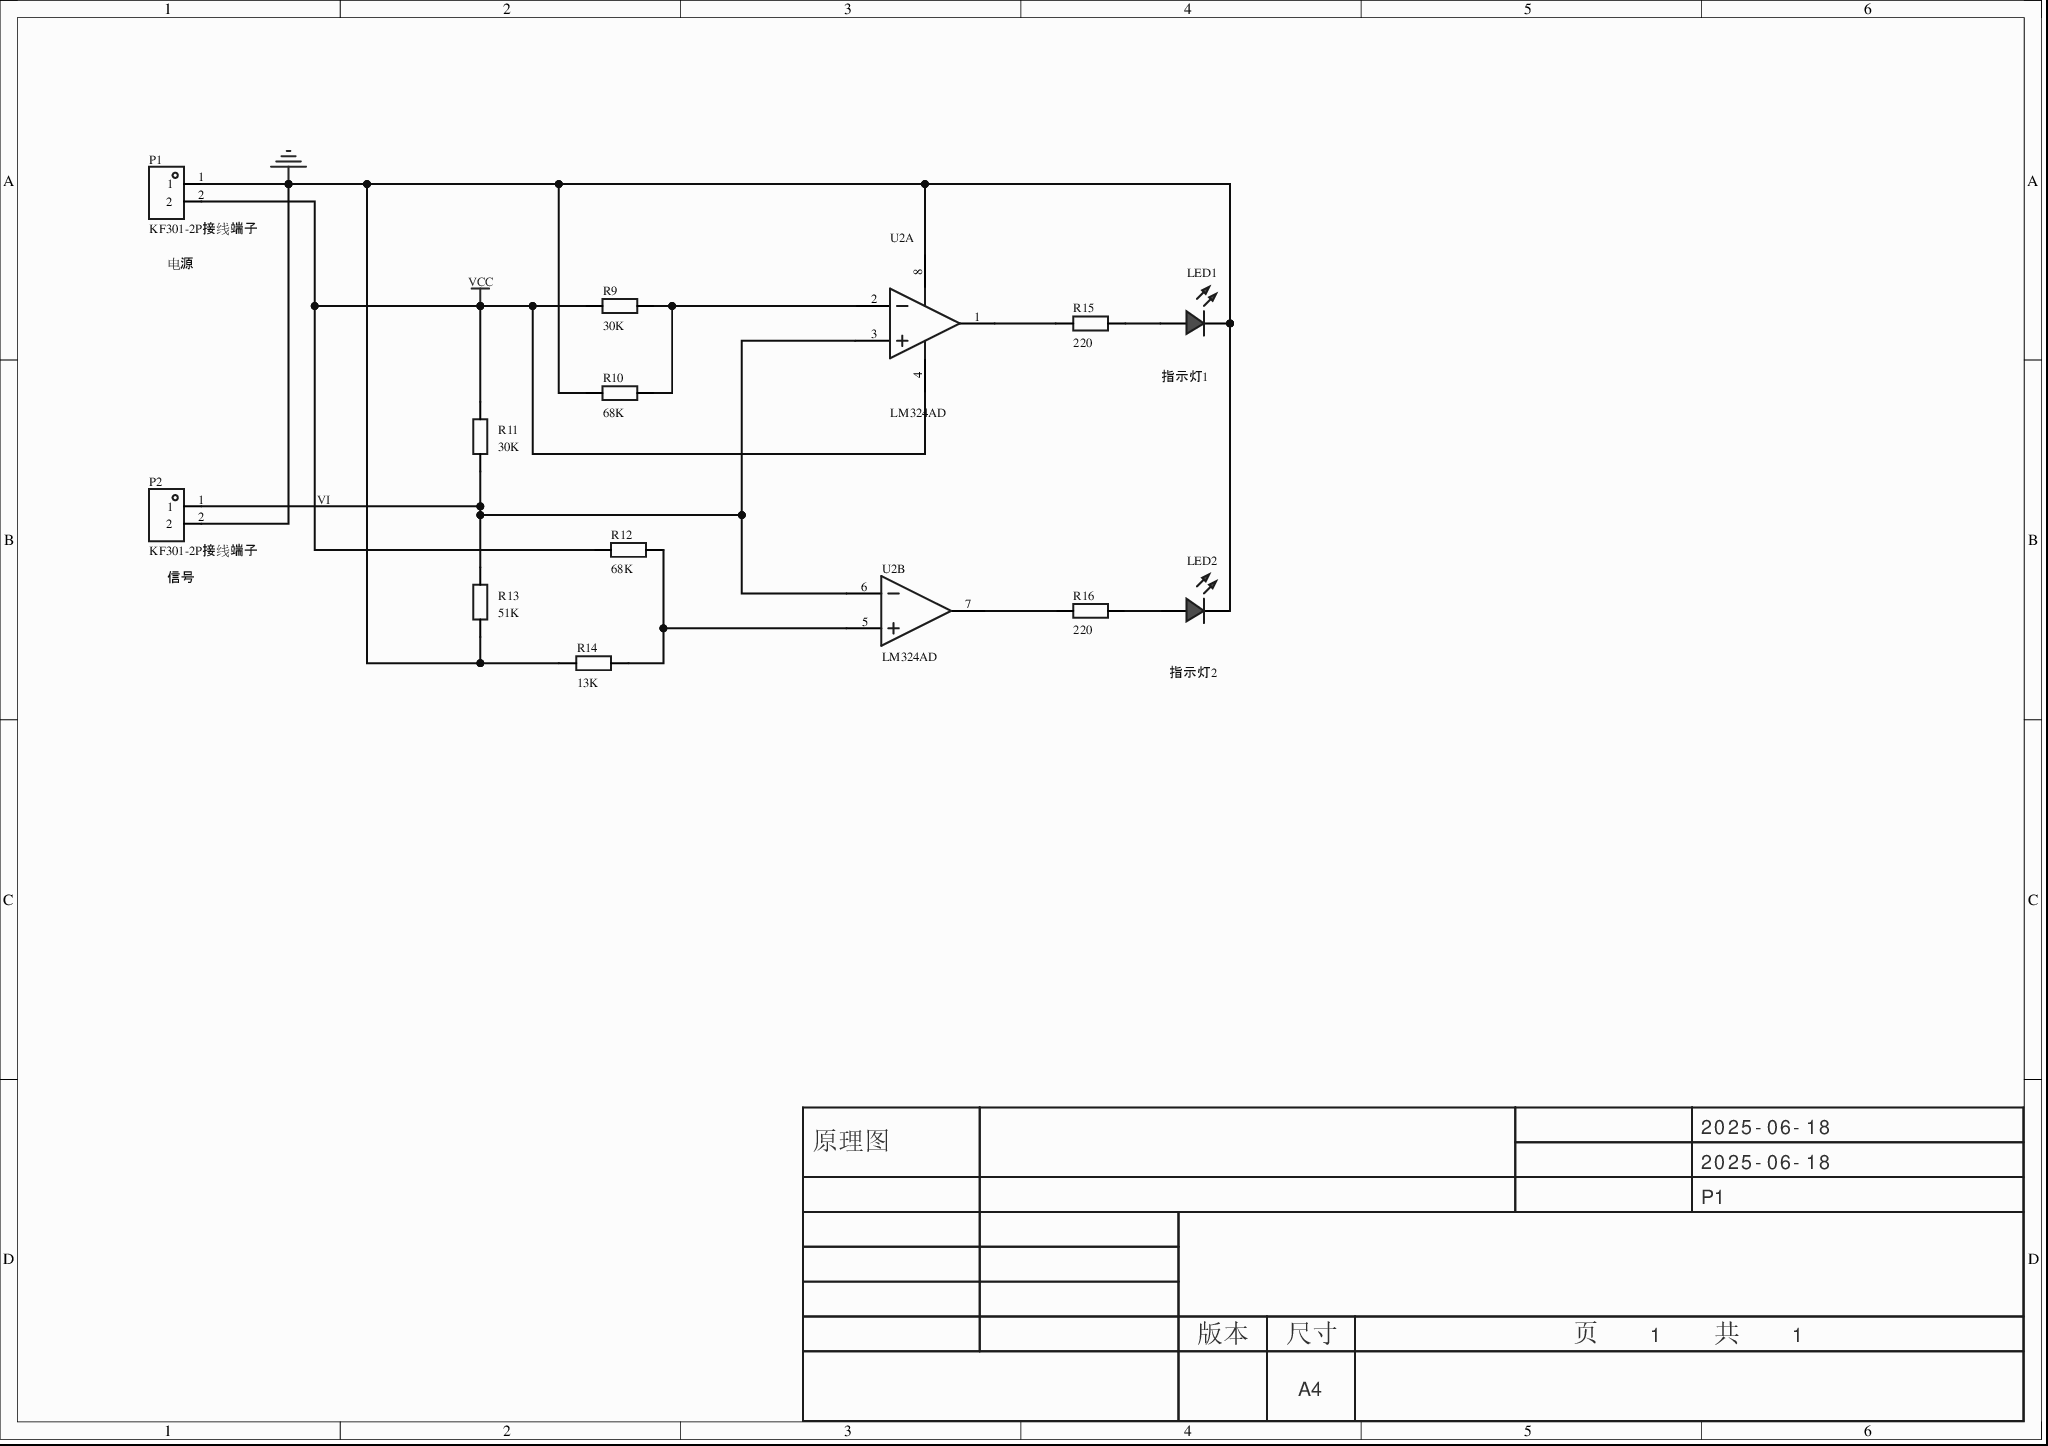
[diagram p0: MISC51032-3.schdoc]
# Altium project MISC51032-2.PrjPcb
1 sheet, 13 parts. Net scope: global (net labels, ports and power ports of the same name join across sheets).
Board file: MISC51032.pcbdoc

## Sheet MISC51032-3.schdoc
size 297 x 209 mm; Version: V1.0; @Project Name: MISC51032; @Page Count: 1; @Update Date: 2025-06-18; @Create Date: 2025-06-18; @Schematic Name: MISC51032; @Page No: 1; @Create Time: 22:04:44; @Update Time: 22:04:48; @Board Name: MISC51032

### Parts
LED1  (no value)  [LED_TH-3mm]
LED2  (no value)  [LED_TH-3mm]
P1  KF301-2P接线端子  [CONN-TH_XY301V-A-5.0-2P]
P2  KF301-2P接线端子  [CONN-TH_XY301V-A-5.0-2P]
R9  30K  [Res_1/8W]
R10  68K  [Res_1/8W]
R11  30K  [Res_1/8W]
R12  68K  [Res_1/8W]
R13  51K  [Res_1/8W]
R14  13K  [Res_1/8W]
R15  220  [Res_1/8W]
R16  220  [Res_1/8W]
U2  LM324AD  [DIP-8_L9.3-W6.4-P2.54-LS7.6-BL]  (parts A,B of 2)

### Nets
GND: LED1.2(A) LED2.2(A) P1.1 P2.2 R10.1 R13.1 R14.1 U2.8(VCC+)
VCC: P1.2 R9.1 R11.2 R12.1 U2.4(VCC-)
VI: P2.1 R11.1 R13.2 U2.3(IN1+) U2.6(IN2-)
NetLED1_1: LED1.1(C) R15.2
NetLED2_1: LED2.1(C) R16.2
NetR9_2: R9.2 R10.2 U2.2(IN1-)
NetR12_2: R12.2 R14.2 U2.5(IN2+)
NetR15_1: R15.1 U2.1(OUT1)
NetR16_1: R16.1 U2.7(OUT2)

### Notes on the sheet
- (near P1) 电源
- 指示灯1
- (near P2) 信号
- 指示灯2
- 2025-06-18
- 原理图
- P1
- 版本
- 尺寸
- A4
- 页    1    共    1

### Library data of the parts
LED1 LED2 = LED_TH-R_3mm: ConvertToPcb: yes; ModelId: a497c992633541038a38947cdc58012f; ModelName: LED-TH-3mm_R; ModelTransform: 141.274,153.327,0,0,0,0,-5.984,0,-137.795; Symbol: LED_TH-R; Device: LED_TH-R_3mm; AddInBom: yes; FootprintName: LED_TH-3mm; Supplier Footprint: 插件
P1 P2 = KF301-2P接线端子: AddInBom: yes; ModelId: ef7ead88b0f2448d904975b26718870f; ModelTransform: 417.322,299.212,0,0,0,0,11.811,-7.835,-157.48; Symbol: KF301-2P接线端子; Device: KF301-2P接线端子; LCSC Part Name: KF301-2P接线端子; SupplierPart: C9900016950; ManufacturerPart: KF301-2P接线端子; Supplier Footprint: CK301-2P; Supplier: LCSC; ConvertToPcb: yes; FootprintName: CONN-TH_XY301V-A-5.0-2P; ModelName: CONN-TH_XY301V-A-5.0-2P
R9-R16 = Res_AXIAL-1/8W: ConvertToPcb: yes; SymbolName: 电阻; ModelId: b2b5ae7ae4c642178fe0039925c86a3f; ModelName: RES-TH_BD1.8-L3.2-P7.20-D0.4; ModelTransform: 282.86,66.88,253.09,0,0,0,0,0,-191; Device: Res_AXIAL-1/8W; AddInBom: yes; Supplier Footprint: 轴向引线; FootprintName: Res_1/8W
  R9 R11: Value: 30K
  R10 R12: Value: 68K
  R13: Value: 51K
  R14: Value: 13K
  R15 R16: Value: 220
U2 = NE5532N: 放大器数:双路;轨到轨:-;增益带宽积(GBP):10MHz;输入失调电压(Vos):5mV;压摆率(SR):11V/us;输入偏置电流(Ib):500nA;; Manufacturer: HGSEMI(华冠); Relevance: []; AddInBom: yes; ModelId: e1ba2ac1384341a197ae27979c8d8942; ModelName: DIP-8_L9.3-W6.4-H4.5-P2.54-LS7.6-BL; ModelTransform: 364.173,311.8104,0,0,0,0,0,0,-118.11; Number of Channels: 双路; Maximum Power Supply Range (Vdd-Vss): 44V; Gain Bandwidth Product: 10MHz; Vos - Input Offset Voltage: 5mV; Slew Rate: 11V/us; Ib - Input Bias Current: 500nA; Input Offset Current(Ios): 200nA; Noise density(eN): 8nV/√Hz@1kHz; Common Mode Rejection Ratio(CMRR): 100dB; Dual Supply: ±22V; Symbol: NE5532N; Manufacturer Part: LM324AD; Device: NE5532N; LCSC Part Name: NE5532N; SupplierPart: C2987282; Supplier Footprint: DIP-8; JLCPCB Part Class: 扩展库; Datasheet: https://atta.szlcsc.com/upload/public/pdf/source/20220420/2D3D2D023E04B50C3DA859F976397601.pdf; Supplier: LCSC; ConvertToPcb: yes; FootprintName: DIP-8_L9.3-W6.4-P2.54-LS7.6-BL; Rail to Rail: -; Input Offset Voltage Drift(Vos TC): -; Input offset current drift(Ios TC): -; Quiescent Current: -; Output Current: -; Operating Temperature: 0℃~+70℃; Single supply: -